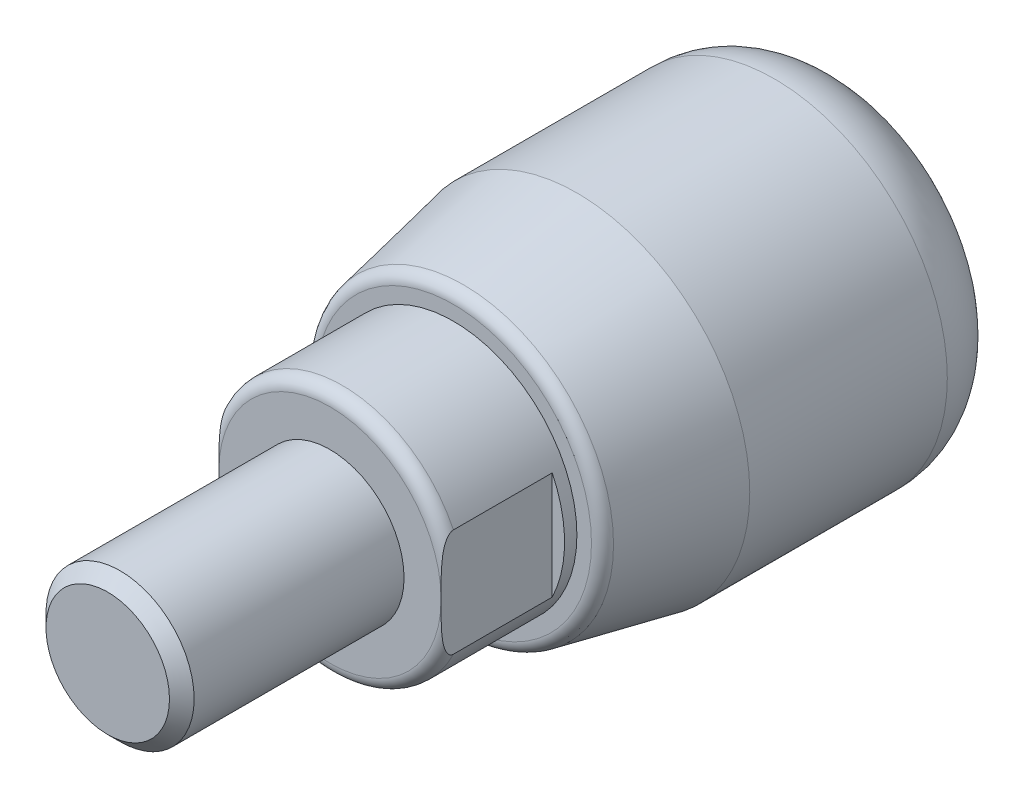
SolidWorks part; units mm, degrees
ref_plane "Front Plane" through (0, 0, 0) normal (0, 0, 1) x (1, 0, 0)
ref_plane "Top Plane" through (0, 0, 0) normal (0, 1, 0) x (1, 0, 0)
ref_plane "Right Plane" through (0, 0, 0) normal (1, 0, 0) x (0, 0, -1)
sketch "Sketch1" plane through (0, 0, 0) normal (0, 0, 1) x (1, 0, 0)
  circle A0 centre (0, 0) radius 7
  dimension "D1" = 14
extrude "Boss-Extrude1" add sketch "Sketch1" along normal mid plane 16
sketch "Sketch2" plane through (0, 0, 8) normal (0, 0, 1) x (1, 0, 0)
  circle A0 centre (0, 0) radius 5
  dimension "D1" = 10
extrude "Boss-Extrude2" add sketch "Sketch2" along normal blind 5
sketch "Sketch3" plane through (0, 0, 13) normal (0, 0, 1) x (1, 0, 0)
  circle A0 centre (0, 0) radius 3
  dimension "D1" = 6
extrude "Boss-Extrude3" add sketch "Sketch3" along normal blind 9
cosmetic thread "Cosmetic Thread1" parameters "D1"=9, "D2"=5
chamfer "Chamfer1" distance 5 distance2 1 1 edges at (7, 0, 8)
fillet "Fillet1" radius 3 1 edges at (7, 0, -8)
fillet "Fillet2" radius 0.5 1 edges at (6, 0, 8)
fillet "Fillet3" radius 0.5 1 edges at (5, 0, 13)
sketch "Sketch4" plane through (0, 0, 13) normal (0, 0, 1) x (1, 0, 0)
  line L1 (-4.5, 5) -> (4.5, 5)
  line L2 (-4.5, 5) -> (-4.5, -5)
  line L3 (-4.5, -5) -> (4.5, -5)
  line L4 (4.5, 5) -> (4.5, -5)
  line L5 (-4.5, 5) -> (4.5, -5) construction
  line L6 (-4.5, -5) -> (4.5, 5) construction
  point P0 (0, 0)
  dimension "D1" = 10
  dimension "D2" = 9
extrude "Cut-Extrude1" cut sketch "Sketch4" against normal blind 4.5 flip side to cut
chamfer "Chamfer3" distance 0.5 angle 45 1 edges at (3, 0, 22)
